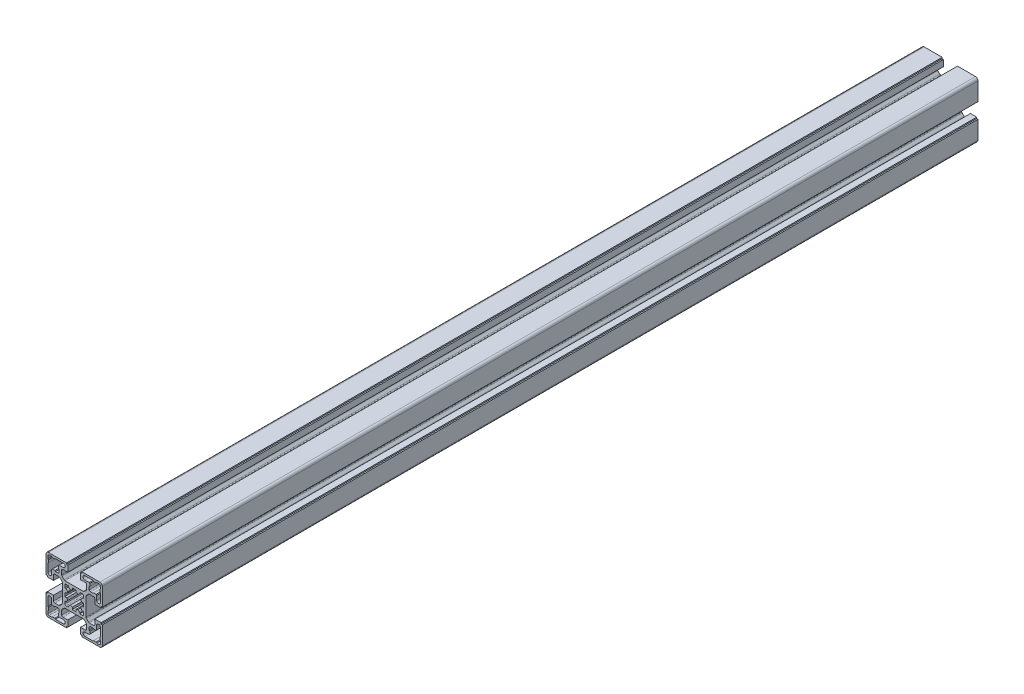
SolidWorks part; units mm, degrees
material "1.11.40.040040.04"
ref_plane "前视基准面" through (0, 0, 0) normal (0, 0, 1) x (1, 0, 0)
ref_plane "上视基准面" through (0, 0, 0) normal (0, 1, 0) x (1, 0, 0)
ref_plane "右视基准面" through (0, 0, 0) normal (1, 0, 0) x (0, 0, -1)
sketch "草图1" plane through (0, 0, 0) normal (0, 0, 1) x (1, 0, 0)
  line L0 (30.535, 44.0271) -> (29.0823, 45.4798)
  line L1 (31.4137, 44.0271) -> (30.535, 44.0271)
  line L2 (31.4137, 42.0271) -> (31.4137, 44.0271)
  line L3 (28.4137, 41.0271) -> (30.4137, 41.0271)
  line L4 (28.4137, 41.9058) -> (28.4137, 41.0271)
  line L5 (26.961, 43.3585) -> (28.4137, 41.9058)
  line L6 (25.4137, 41.0271) -> (25.4137, 42.7176)
  line L7 (22.4137, 41.0271) -> (25.4137, 41.0271)
  line L8 (22.4137, 42.7176) -> (22.4137, 41.0271)
  line L9 (19.4137, 41.9058) -> (20.8664, 43.3585)
  line L10 (19.4137, 41.0271) -> (19.4137, 41.9058)
  line L11 (17.4137, 41.0271) -> (19.4137, 41.0271)
  line L12 (16.4137, 44.0271) -> (16.4137, 42.0271)
  line L13 (17.2924, 44.0271) -> (16.4137, 44.0271)
  line L14 (18.7451, 45.4798) -> (17.2924, 44.0271)
  line L15 (16.4137, 47.0271) -> (18.1042, 47.0271)
  line L16 (16.4137, 50.0271) -> (16.4137, 47.0271)
  line L17 (18.1042, 50.0271) -> (16.4137, 50.0271)
  line L18 (17.2924, 53.0271) -> (18.7451, 51.5744)
  line L19 (16.4137, 53.0271) -> (17.2924, 53.0271)
  line L20 (16.4137, 55.0271) -> (16.4137, 53.0271)
  line L21 (19.4137, 56.0271) -> (17.4137, 56.0271)
  line L22 (19.4137, 55.1484) -> (19.4137, 56.0271)
  line L23 (20.8664, 53.6957) -> (19.4137, 55.1484)
  line L24 (22.4137, 56.0271) -> (22.4137, 54.3366)
  line L25 (25.4137, 56.0271) -> (22.4137, 56.0271)
  line L26 (25.4137, 54.3366) -> (25.4137, 56.0271)
  line L27 (28.4137, 55.1484) -> (26.961, 53.6957)
  line L28 (28.4137, 56.0271) -> (28.4137, 55.1484)
  line L29 (30.4137, 56.0271) -> (28.4137, 56.0271)
  line L30 (31.4137, 53.0271) -> (31.4137, 55.0271)
  line L31 (30.535, 53.0271) -> (31.4137, 53.0271)
  line L32 (29.0823, 51.5744) -> (30.535, 53.0271)
  line L33 (31.4137, 50.0271) -> (29.7232, 50.0271)
  line L34 (31.4137, 47.0271) -> (31.4137, 50.0271)
  line L35 (29.7232, 47.0271) -> (31.4137, 47.0271)
  line L36 (11.4137, 66.0271) -> (11.9137, 66.5271)
  line L37 (11.4137, 64.0271) -> (11.4137, 66.0271)
  line L38 (11.9137, 63.5271) -> (11.4137, 64.0271)
  line L39 (11.9137, 61.5271) -> (11.9137, 63.5271)
  line L40 (8.9137, 60.5271) -> (10.9137, 60.5271)
  line L41 (8.4137, 61.0271) -> (8.9137, 60.5271)
  line L42 (6.4137, 61.0271) -> (8.4137, 61.0271)
  line L43 (5.9137, 60.5271) -> (6.4137, 61.0271)
  line L44 (5.9137, 57.1271) -> (5.9137, 60.5271)
  line L45 (2.9137, 63.5271) -> (2.9137, 57.1271)
  line L46 (3.4137, 64.0271) -> (2.9137, 63.5271)
  line L47 (3.4137, 66.0271) -> (3.4137, 64.0271)
  line L48 (2.9137, 66.5271) -> (3.4137, 66.0271)
  line L49 (2.9137, 68.5271) -> (2.9137, 66.5271)
  line L50 (5.9137, 69.5271) -> (3.9137, 69.5271)
  line L51 (6.4137, 69.0271) -> (5.9137, 69.5271)
  line L52 (8.4137, 69.0271) -> (6.4137, 69.0271)
  line L53 (8.9137, 69.5271) -> (8.4137, 69.0271)
  line L54 (15.3137, 69.5271) -> (8.9137, 69.5271)
  line L55 (11.9137, 66.5271) -> (15.3137, 66.5271)
  line L56 (11.9137, 30.5271) -> (11.4137, 31.0271)
  line L57 (15.3137, 30.5271) -> (11.9137, 30.5271)
  line L58 (8.9137, 27.5271) -> (15.3137, 27.5271)
  line L59 (8.4137, 28.0271) -> (8.9137, 27.5271)
  line L60 (6.4137, 28.0271) -> (8.4137, 28.0271)
  line L61 (5.9137, 27.5271) -> (6.4137, 28.0271)
  line L62 (3.9137, 27.5271) -> (5.9137, 27.5271)
  line L63 (2.9137, 30.5271) -> (2.9137, 28.5271)
  line L64 (3.4137, 31.0271) -> (2.9137, 30.5271)
  line L65 (3.4137, 33.0271) -> (3.4137, 31.0271)
  line L66 (2.9137, 33.5271) -> (3.4137, 33.0271)
  line L67 (2.9137, 39.9271) -> (2.9137, 33.5271)
  line L68 (5.9137, 36.5271) -> (5.9137, 39.9271)
  line L69 (6.4137, 36.0271) -> (5.9137, 36.5271)
  line L70 (8.4137, 36.0271) -> (6.4137, 36.0271)
  line L71 (8.9137, 36.5271) -> (8.4137, 36.0271)
  line L72 (10.9137, 36.5271) -> (8.9137, 36.5271)
  line L73 (11.9137, 33.5271) -> (11.9137, 35.5271)
  line L74 (11.4137, 33.0271) -> (11.9137, 33.5271)
  line L75 (11.4137, 31.0271) -> (11.4137, 33.0271)
  line L76 (41.9137, 36.5271) -> (41.4137, 36.0271)
  line L77 (41.9137, 39.9271) -> (41.9137, 36.5271)
  line L78 (44.9137, 33.5271) -> (44.9137, 39.9271)
  line L79 (44.4137, 33.0271) -> (44.9137, 33.5271)
  line L80 (44.4137, 31.0271) -> (44.4137, 33.0271)
  line L81 (44.9137, 30.5271) -> (44.4137, 31.0271)
  line L82 (44.9137, 28.5271) -> (44.9137, 30.5271)
  line L83 (41.9137, 27.5271) -> (43.9137, 27.5271)
  line L84 (41.4137, 28.0271) -> (41.9137, 27.5271)
  line L85 (39.4137, 28.0271) -> (41.4137, 28.0271)
  line L86 (38.9137, 27.5271) -> (39.4137, 28.0271)
  line L87 (32.5137, 27.5271) -> (38.9137, 27.5271)
  line L88 (35.9137, 30.5271) -> (32.5137, 30.5271)
  line L89 (36.4137, 31.0271) -> (35.9137, 30.5271)
  line L90 (36.4137, 33.0271) -> (36.4137, 31.0271)
  line L91 (35.9137, 33.5271) -> (36.4137, 33.0271)
  line L92 (35.9137, 35.5271) -> (35.9137, 33.5271)
  line L93 (38.9137, 36.5271) -> (36.9137, 36.5271)
  line L94 (39.4137, 36.0271) -> (38.9137, 36.5271)
  line L95 (41.4137, 36.0271) -> (39.4137, 36.0271)
  line L96 (35.9137, 66.5271) -> (36.4137, 66.0271)
  line L97 (32.5137, 66.5271) -> (35.9137, 66.5271)
  line L98 (38.9137, 69.5271) -> (32.5137, 69.5271)
  line L99 (39.4137, 69.0271) -> (38.9137, 69.5271)
  line L100 (41.4137, 69.0271) -> (39.4137, 69.0271)
  line L101 (41.9137, 69.5271) -> (41.4137, 69.0271)
  line L102 (43.9137, 69.5271) -> (41.9137, 69.5271)
  line L103 (44.9137, 66.5271) -> (44.9137, 68.5271)
  line L104 (44.4137, 66.0271) -> (44.9137, 66.5271)
  line L105 (44.4137, 64.0271) -> (44.4137, 66.0271)
  line L106 (44.9137, 63.5271) -> (44.4137, 64.0271)
  line L107 (44.9137, 57.1271) -> (44.9137, 63.5271)
  line L108 (41.9137, 60.5271) -> (41.9137, 57.1271)
  line L109 (41.4137, 61.0271) -> (41.9137, 60.5271)
  line L110 (39.4137, 61.0271) -> (41.4137, 61.0271)
  line L111 (38.9137, 60.5271) -> (39.4137, 61.0271)
  line L112 (36.9137, 60.5271) -> (38.9137, 60.5271)
  line L113 (35.9137, 63.5271) -> (35.9137, 61.5271)
  line L114 (36.4137, 64.0271) -> (35.9137, 63.5271)
  line L115 (36.4137, 66.0271) -> (36.4137, 64.0271)
  line L116 (33.7066, 40.502) -> (35.3886, 38.82)
  line L117 (33.4137, 55.8451) -> (33.4137, 41.2091)
  line L118 (35.3886, 58.2342) -> (33.7066, 56.5522)
  line L119 (39.4137, 58.5271) -> (36.0957, 58.5271)
  line L120 (40.4137, 53.6271) -> (40.4137, 57.5271)
  line L121 (45.4137, 53.6271) -> (40.4137, 53.6271)
  line L122 (45.4137, 54.6271) -> (45.4137, 53.6271)
  line L123 (46.4137, 54.6271) -> (45.4137, 54.6271)
  line L124 (46.4137, 69.0271) -> (46.4137, 54.6271)
  line L125 (30.0137, 71.0271) -> (44.4137, 71.0271)
  line L126 (30.0137, 70.0271) -> (30.0137, 71.0271)
  line L127 (29.0137, 70.0271) -> (30.0137, 70.0271)
  line L128 (29.0137, 65.0271) -> (29.0137, 70.0271)
  line L129 (32.9137, 65.0271) -> (29.0137, 65.0271)
  line L130 (33.9137, 60.7091) -> (33.9137, 64.0271)
  line L131 (31.9388, 58.32) -> (33.6208, 60.002)
  line L132 (16.5957, 58.0271) -> (31.2317, 58.0271)
  line L133 (14.2066, 60.002) -> (15.8886, 58.32)
  line L134 (13.9137, 64.0271) -> (13.9137, 60.7091)
  line L135 (18.8137, 65.0271) -> (14.9137, 65.0271)
  line L136 (18.8137, 70.0271) -> (18.8137, 65.0271)
  line L137 (17.8137, 70.0271) -> (18.8137, 70.0271)
  line L138 (17.8137, 71.0271) -> (17.8137, 70.0271)
  line L139 (3.4137, 71.0271) -> (17.8137, 71.0271)
  line L140 (1.4137, 54.6271) -> (1.4137, 69.0271)
  line L141 (2.4137, 54.6271) -> (1.4137, 54.6271)
  line L142 (2.4137, 53.6271) -> (2.4137, 54.6271)
  line L143 (7.4137, 53.6271) -> (2.4137, 53.6271)
  line L144 (7.4137, 57.5271) -> (7.4137, 53.6271)
  line L145 (11.7317, 58.5271) -> (8.4137, 58.5271)
  line L146 (14.1208, 56.5522) -> (12.4388, 58.2342)
  line L147 (14.4137, 41.2091) -> (14.4137, 55.8451)
  line L148 (12.4388, 38.82) -> (14.1208, 40.502)
  line L149 (8.4137, 38.5271) -> (11.7317, 38.5271)
  line L150 (7.4137, 43.4271) -> (7.4137, 39.5271)
  line L151 (2.4137, 43.4271) -> (7.4137, 43.4271)
  line L152 (2.4137, 42.4271) -> (2.4137, 43.4271)
  line L153 (1.4137, 42.4271) -> (2.4137, 42.4271)
  line L154 (1.4137, 28.0271) -> (1.4137, 42.4271)
  line L155 (17.8137, 26.0271) -> (3.4137, 26.0271)
  line L156 (17.8137, 27.0271) -> (17.8137, 26.0271)
  line L157 (18.8137, 27.0271) -> (17.8137, 27.0271)
  line L158 (18.8137, 32.0271) -> (18.8137, 27.0271)
  line L159 (14.9137, 32.0271) -> (18.8137, 32.0271)
  line L160 (13.9137, 36.3451) -> (13.9137, 33.0271)
  line L161 (15.8886, 38.7342) -> (14.2066, 37.0522)
  line L162 (31.2317, 39.0271) -> (16.5957, 39.0271)
  line L163 (33.6208, 37.0522) -> (31.9388, 38.7342)
  line L164 (33.9137, 33.0271) -> (33.9137, 36.3451)
  line L165 (29.0137, 32.0271) -> (32.9137, 32.0271)
  line L166 (29.0137, 27.0271) -> (29.0137, 32.0271)
  line L167 (30.0137, 27.0271) -> (29.0137, 27.0271)
  line L168 (30.0137, 26.0271) -> (30.0137, 27.0271)
  line L169 (44.4137, 26.0271) -> (30.0137, 26.0271)
  line L170 (46.4137, 42.4271) -> (46.4137, 28.0271)
  line L171 (45.4137, 42.4271) -> (46.4137, 42.4271)
  line L172 (45.4137, 43.4271) -> (45.4137, 42.4271)
  line L173 (40.4137, 43.4271) -> (45.4137, 43.4271)
  line L174 (40.4137, 39.5271) -> (40.4137, 43.4271)
  line L175 (36.0957, 38.5271) -> (39.4137, 38.5271)
  arc A0 (30.4137, 41.0271) -> (31.4137, 42.0271) centre (30.4137, 42.0271) ccw
  arc A1 (25.4137, 42.7176) -> (26.961, 43.3585) centre (23.9137, 48.5271) ccw
  arc A2 (20.8664, 43.3585) -> (22.4137, 42.7176) centre (23.9137, 48.5271) ccw
  arc A3 (16.4137, 42.0271) -> (17.4137, 41.0271) centre (17.4137, 42.0271) ccw
  arc A4 (18.1042, 47.0271) -> (18.7451, 45.4798) centre (23.9137, 48.5271) ccw
  arc A5 (18.7451, 51.5744) -> (18.1042, 50.0271) centre (23.9137, 48.5271) ccw
  arc A6 (17.4137, 56.0271) -> (16.4137, 55.0271) centre (17.4137, 55.0271) ccw
  arc A7 (22.4137, 54.3366) -> (20.8664, 53.6957) centre (23.9137, 48.5271) ccw
  arc A8 (26.961, 53.6957) -> (25.4137, 54.3366) centre (23.9137, 48.5271) ccw
  arc A9 (31.4137, 55.0271) -> (30.4137, 56.0271) centre (30.4137, 55.0271) ccw
  arc A10 (29.7232, 50.0271) -> (29.0823, 51.5744) centre (23.9137, 48.5271) ccw
  arc A11 (29.0823, 45.4798) -> (29.7232, 47.0271) centre (23.9137, 48.5271) ccw
  arc A12 (10.9137, 60.5271) -> (11.9137, 61.5271) centre (10.9137, 61.5271) ccw
  arc A13 (2.9137, 57.1271) -> (5.9137, 57.1271) centre (4.4137, 57.1271) ccw
  arc A14 (3.9137, 69.5271) -> (2.9137, 68.5271) centre (3.9137, 68.5271) ccw
  arc A15 (15.3137, 66.5271) -> (15.3137, 69.5271) centre (15.3137, 68.0271) ccw
  arc A16 (15.3137, 27.5271) -> (15.3137, 30.5271) centre (15.3137, 29.0271) ccw
  arc A17 (2.9137, 28.5271) -> (3.9137, 27.5271) centre (3.9137, 28.5271) ccw
  arc A18 (5.9137, 39.9271) -> (2.9137, 39.9271) centre (4.4137, 39.9271) ccw
  arc A19 (11.9137, 35.5271) -> (10.9137, 36.5271) centre (10.9137, 35.5271) ccw
  arc A20 (44.9137, 39.9271) -> (41.9137, 39.9271) centre (43.4137, 39.9271) ccw
  arc A21 (43.9137, 27.5271) -> (44.9137, 28.5271) centre (43.9137, 28.5271) ccw
  arc A22 (32.5137, 30.5271) -> (32.5137, 27.5271) centre (32.5137, 29.0271) ccw
  arc A23 (36.9137, 36.5271) -> (35.9137, 35.5271) centre (36.9137, 35.5271) ccw
  arc A24 (32.5137, 69.5271) -> (32.5137, 66.5271) centre (32.5137, 68.0271) ccw
  arc A25 (44.9137, 68.5271) -> (43.9137, 69.5271) centre (43.9137, 68.5271) ccw
  arc A26 (41.9137, 57.1271) -> (44.9137, 57.1271) centre (43.4137, 57.1271) ccw
  arc A27 (35.9137, 61.5271) -> (36.9137, 60.5271) centre (36.9137, 61.5271) ccw
  arc A28 (35.3886, 38.82) -> (36.0957, 38.5271) centre (36.0957, 39.5271) ccw
  arc A29 (33.4137, 41.2091) -> (33.7066, 40.502) centre (34.4137, 41.2091) ccw
  arc A30 (33.7066, 56.5522) -> (33.4137, 55.8451) centre (34.4137, 55.8451) ccw
  arc A31 (36.0957, 58.5271) -> (35.3886, 58.2342) centre (36.0957, 57.5271) ccw
  arc A32 (40.4137, 57.5271) -> (39.4137, 58.5271) centre (39.4137, 57.5271) ccw
  arc A33 (46.4137, 69.0271) -> (44.4137, 71.0271) centre (44.4137, 69.0271) ccw
  arc A34 (33.9137, 64.0271) -> (32.9137, 65.0271) centre (32.9137, 64.0271) ccw
  arc A35 (33.6208, 60.002) -> (33.9137, 60.7091) centre (32.9137, 60.7091) ccw
  arc A36 (31.2317, 58.0271) -> (31.9388, 58.32) centre (31.2317, 59.0271) ccw
  arc A37 (15.8886, 58.32) -> (16.5957, 58.0271) centre (16.5957, 59.0271) ccw
  arc A38 (13.9137, 60.7091) -> (14.2066, 60.002) centre (14.9137, 60.7091) ccw
  arc A39 (14.9137, 65.0271) -> (13.9137, 64.0271) centre (14.9137, 64.0271) ccw
  arc A40 (3.4137, 71.0271) -> (1.4137, 69.0271) centre (3.4137, 69.0271) ccw
  arc A41 (8.4137, 58.5271) -> (7.4137, 57.5271) centre (8.4137, 57.5271) ccw
  arc A42 (12.4388, 58.2342) -> (11.7317, 58.5271) centre (11.7317, 57.5271) ccw
  arc A43 (14.4137, 55.8451) -> (14.1208, 56.5522) centre (13.4137, 55.8451) ccw
  arc A44 (14.1208, 40.502) -> (14.4137, 41.2091) centre (13.4137, 41.2091) ccw
  arc A45 (11.7317, 38.5271) -> (12.4388, 38.82) centre (11.7317, 39.5271) ccw
  arc A46 (7.4137, 39.5271) -> (8.4137, 38.5271) centre (8.4137, 39.5271) ccw
  arc A47 (1.4137, 28.0271) -> (3.4137, 26.0271) centre (3.4137, 28.0271) ccw
  arc A48 (13.9137, 33.0271) -> (14.9137, 32.0271) centre (14.9137, 33.0271) ccw
  arc A49 (14.2066, 37.0522) -> (13.9137, 36.3451) centre (14.9137, 36.3451) ccw
  arc A50 (16.5957, 39.0271) -> (15.8886, 38.7342) centre (16.5957, 38.0271) ccw
  arc A51 (31.9388, 38.7342) -> (31.2317, 39.0271) centre (31.2317, 38.0271) ccw
  arc A52 (33.9137, 36.3451) -> (33.6208, 37.0522) centre (32.9137, 36.3451) ccw
  arc A53 (32.9137, 32.0271) -> (33.9137, 33.0271) centre (32.9137, 33.0271) ccw
  arc A54 (44.4137, 26.0271) -> (46.4137, 28.0271) centre (44.4137, 28.0271) ccw
  arc A55 (39.4137, 38.5271) -> (40.4137, 39.5271) centre (39.4137, 39.5271) ccw
extrude "拉伸1" add sketch "草图1" along normal blind 700
